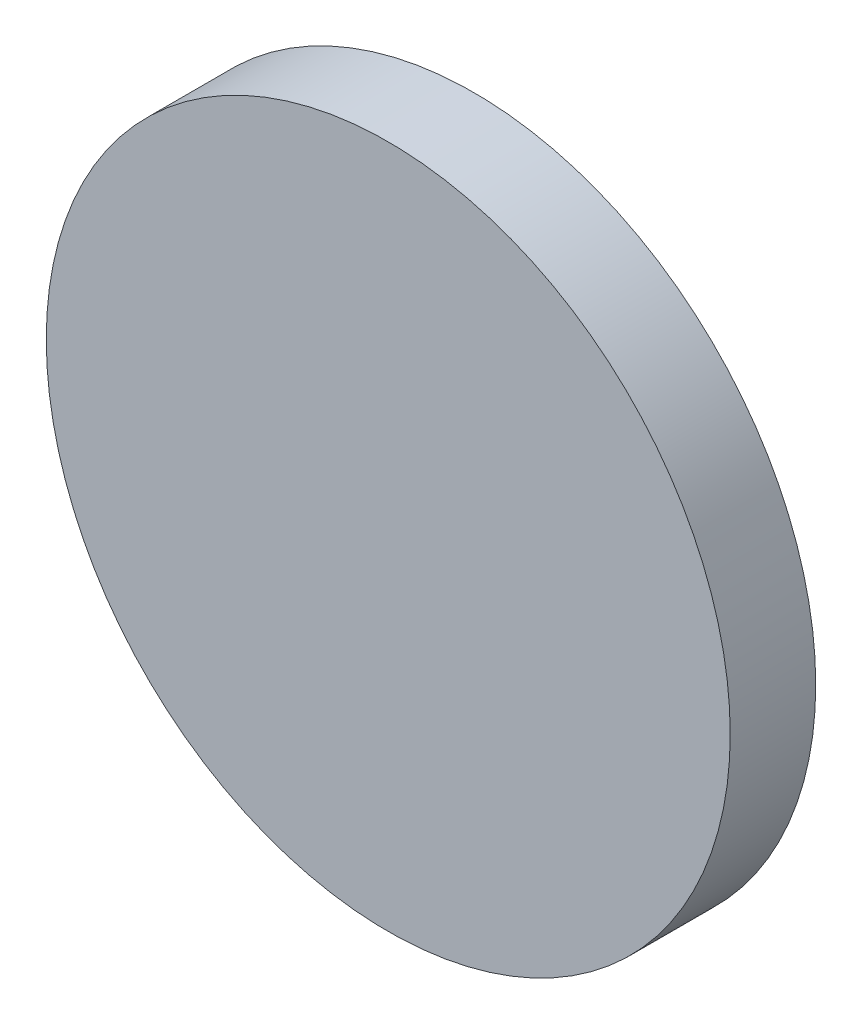
SolidWorks part; units mm, degrees
ref_plane "Front Plane" through (0, 0, 0) normal (0, 0, 1) x (1, 0, 0)
ref_plane "Top Plane" through (0, 0, 0) normal (0, 1, 0) x (1, 0, 0)
ref_plane "Right Plane" through (0, 0, 0) normal (1, 0, 0) x (0, 0, -1)
sketch "Sketch1" plane through (0, 0, 0) normal (0, 0, 1) x (1, 0, 0)
  circle A1 centre (0, 0) radius 30
  circle A2 centre (0, 0) radius 30
  dimension "D1" = 0
extrude "Boss-Extrude1" add sketch "Sketch1" along normal blind 7.5
